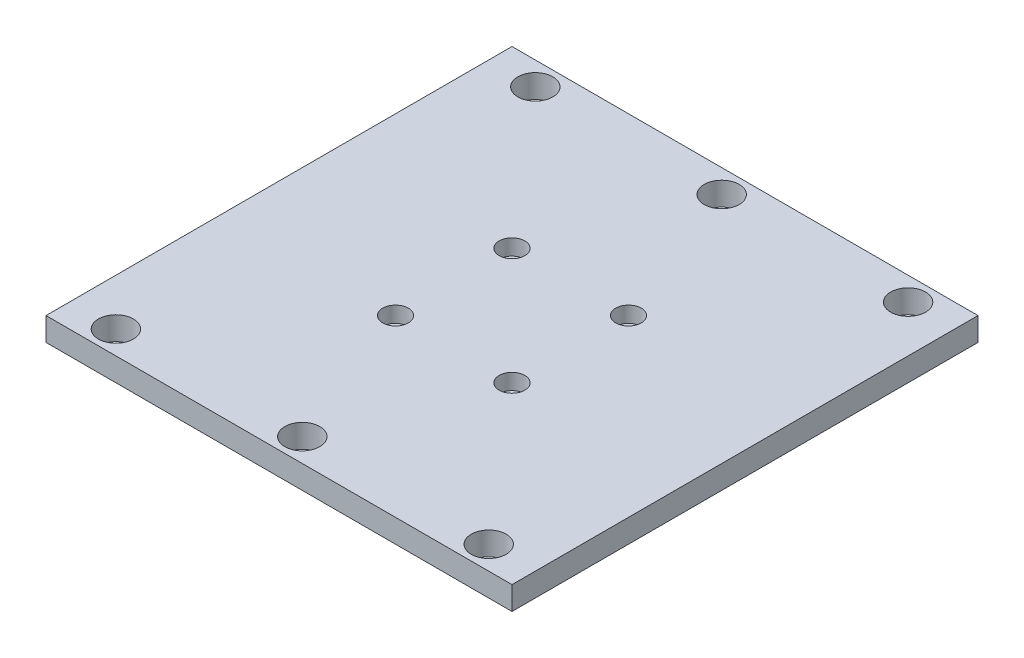
from build123d import *

# Parameters (mm, degrees)
SKETCH1_W                                           = 200
SKETCH1_H                                           = 200
BOSS_EXTRUDE1_DEPTH                                 = 5
SKETCH2_R                                           = 7.5
CUT_EXTRUDE1_DEPTH                                  = 10
LPATTERN1_COUNT                                     = 2
LPATTERN1_PITCH                                     = 180
LPATTERN1_COUNT_DIR2                                = 3
LPATTERN1_PITCH_DIR2                                = 80
HOLE_SIZE_BASED_ON_SOCKET_HEAD_CAP_SCRE_D           = 6.6
HOLE_SIZE_BASED_ON_SOCKET_HEAD_CAP_SCRE_CBORE_D     = 11
HOLE_SIZE_BASED_ON_SOCKET_HEAD_CAP_SCRE_CBORE_DEPTH = 6.8


with BuildPart() as part:
    # Sketch1 → Boss-Extrude1 (new, symmetric)
    with BuildSketch(Plane(origin=(0, 0, 0), x_dir=(1, 0, 0), z_dir=(0, 1, 0))):
        Rectangle(SKETCH1_W, SKETCH1_H)
    extrude(amount=BOSS_EXTRUDE1_DEPTH, both=True)

    # Sketch2 → Cut-Extrude1 (cut)
    with BuildSketch(Plane(origin=(0, 5, 0), x_dir=(1, 0, 0), z_dir=(0, 1, 0))):
        with Locations(Location((80, 90, 0), (0, 0, 270))):
            Circle(SKETCH2_R)
    cut_extrude1 = extrude(amount=-CUT_EXTRUDE1_DEPTH, mode=Mode.SUBTRACT)

    # LPattern1: Cut-Extrude1 2 × 3
    with Locations(*[(-j * LPATTERN1_PITCH_DIR2, 0, i * LPATTERN1_PITCH) for i in range(LPATTERN1_COUNT) for j in range(LPATTERN1_COUNT_DIR2) if (i, j) != (0, 0)]):
        add(cut_extrude1, mode=Mode.SUBTRACT)

    # Hole Size (based on socket head cap screw type)1 (through all)
    with Locations(Plane(origin=(0, 5, 0), x_dir=(1, 0, 0), z_dir=(0, 1, 0))):
        with Locations((25, 25), (25, -25), (-25, 25), (-25, -25)):
            CounterBoreHole(HOLE_SIZE_BASED_ON_SOCKET_HEAD_CAP_SCRE_D / 2, HOLE_SIZE_BASED_ON_SOCKET_HEAD_CAP_SCRE_CBORE_D / 2, HOLE_SIZE_BASED_ON_SOCKET_HEAD_CAP_SCRE_CBORE_DEPTH)


solid = part.part
